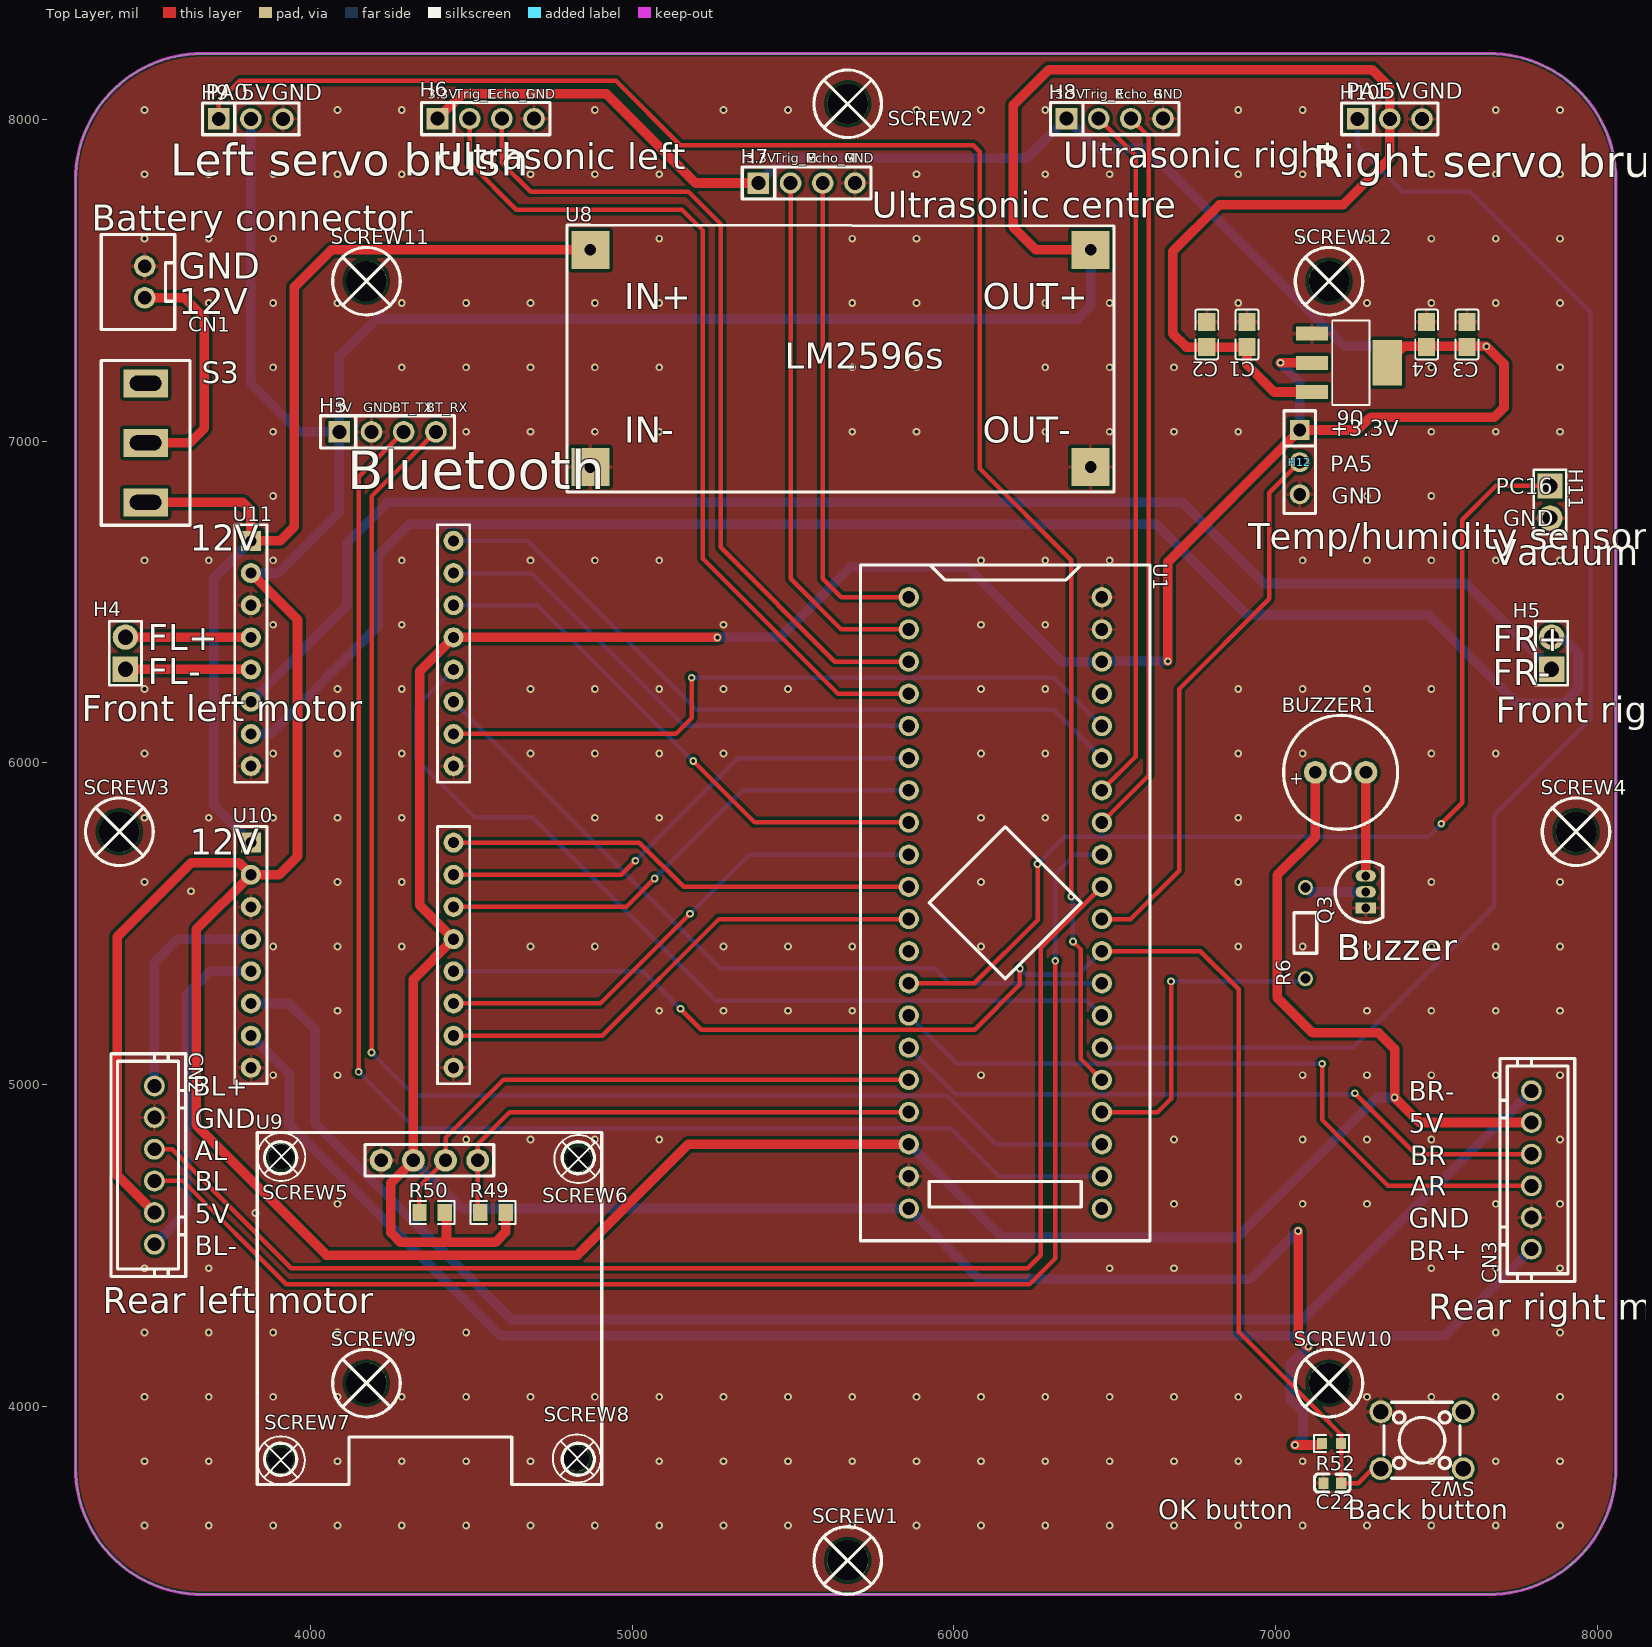
[diagram p0: Top Layer view]
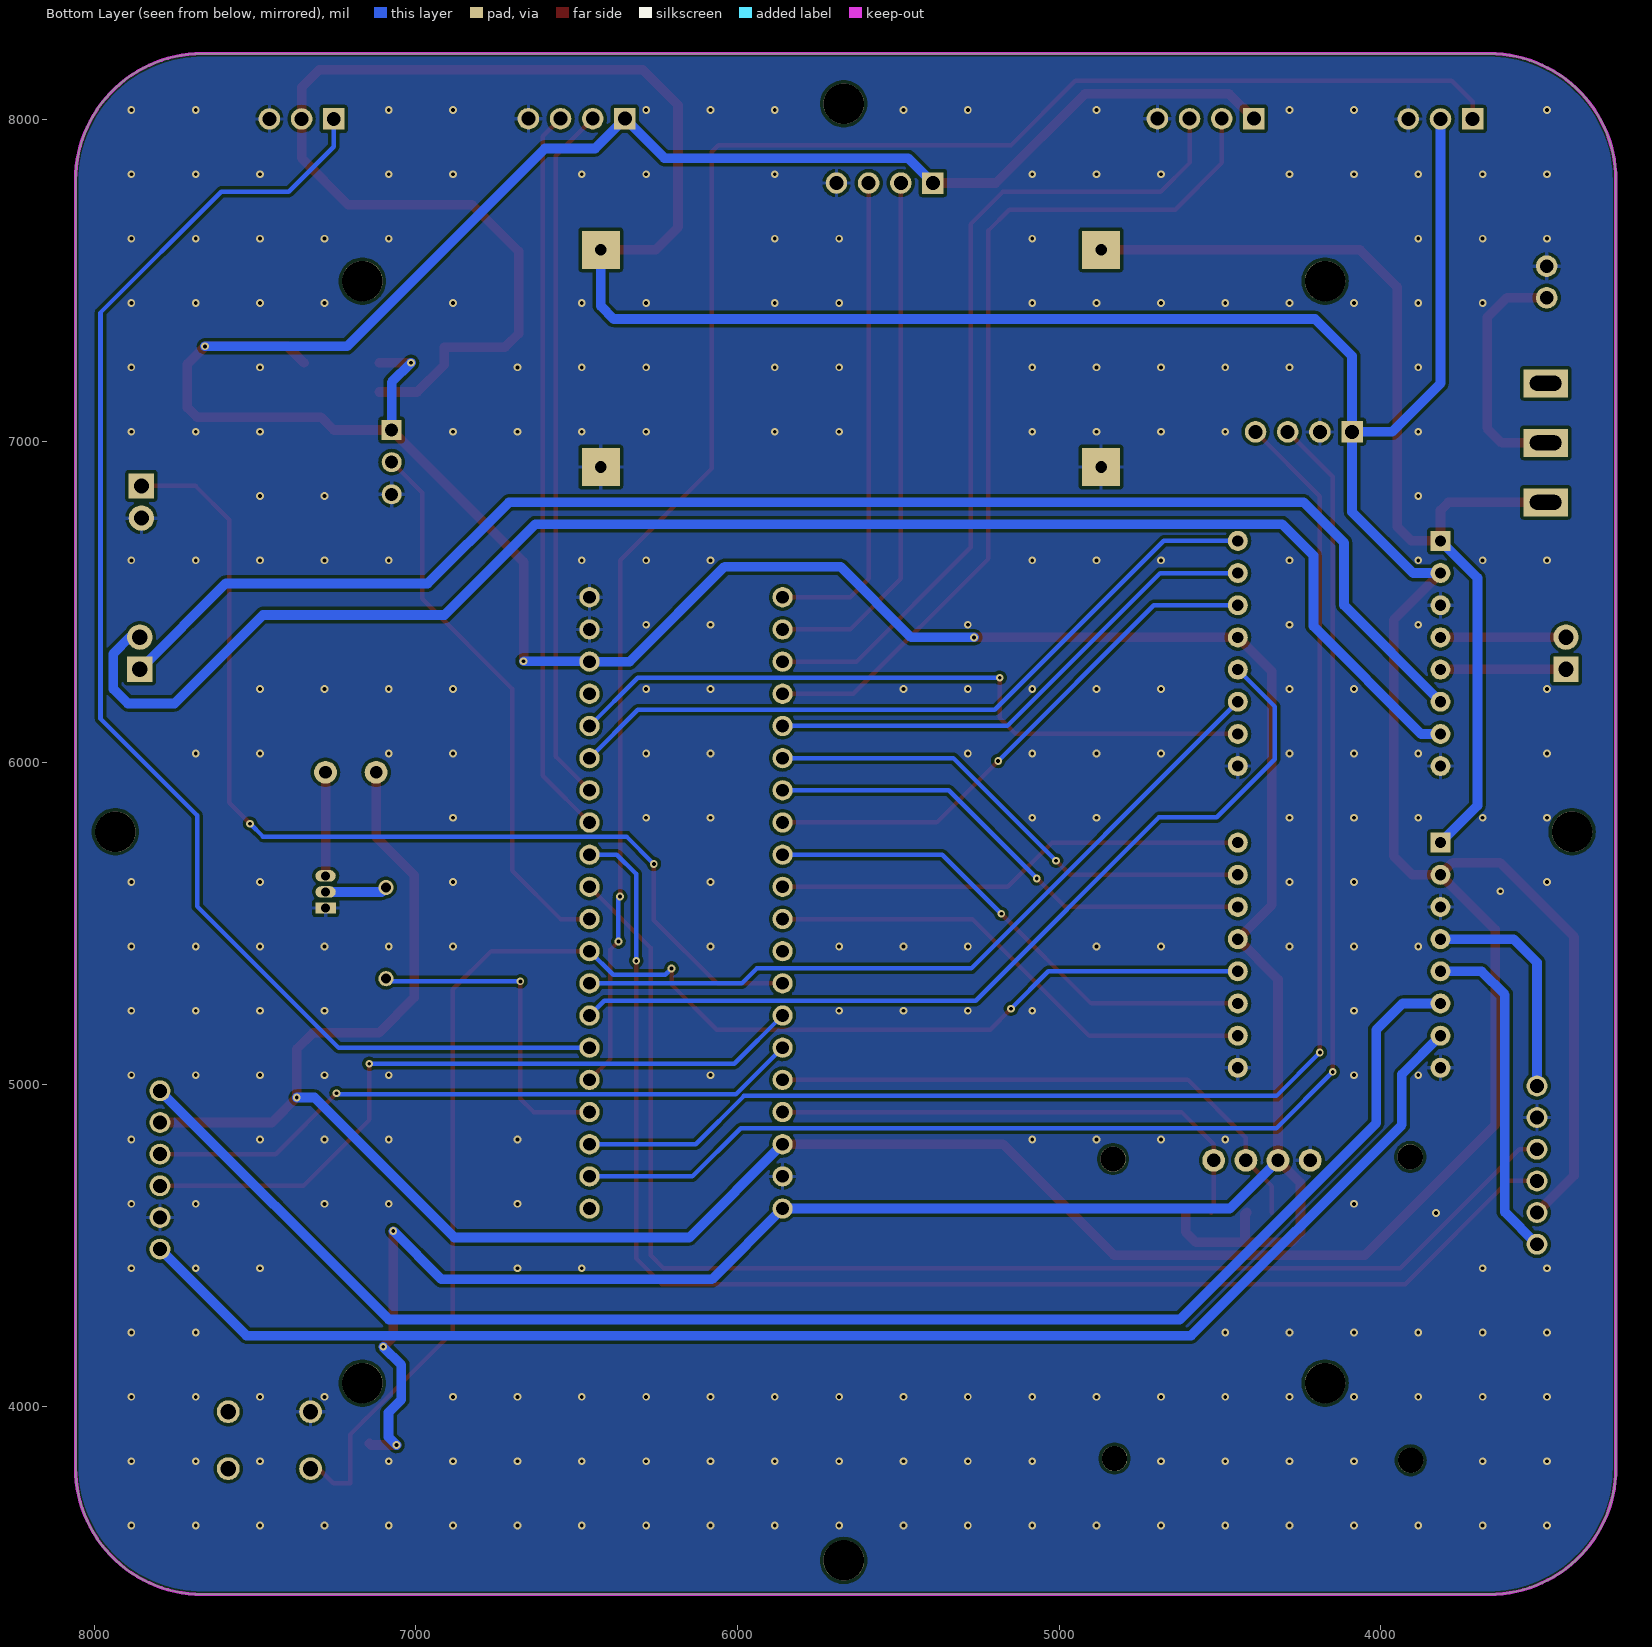
[diagram p1: Bottom Layer view, seen from below]
# Altium PCB MISC49897.pcbdoc
Units mil, origin at the board's own origin, x right, y up, seen from the top; angles counter-clockwise.
Board outline 4787.56 x 4789.41 mil, 2 copper layers (Top Layer, Bottom Layer), stack 62.206 mil thick; 44 components, 49 nets, 171 pads, 306 vias.

## Layer stack, top to bottom
Top Solder Mask Layer: solder mask 0.394, Dk 3.3
Top Layer: signal copper 1.379
Dielectric1: surface 59.449, FR4, Dk 4.5
Bottom Layer: signal copper 1.378
Bottom Solder Mask Layer: solder mask 0.394, Dk 3.3

## Board outline
3663.7,8205 ccw(c3663.7,7811.3) 3270,7811.3 3270,3809.29 ccw(c3663.7,3809.29) 3663.7,3415.59 7663.86,3415.59 ccw(c7663.86,3809.29) 8057.56,3809.29 8057.56,7811.3 ccw(c7663.86,7811.3) 7663.86,8205

## Design rules (kind name [scope] priority, off if disabled: settings)
BoardOutlineClearance copperThickness2oz_1 [All] p2 off: genericclearance=7.99 ignorepadtopadclearanceinfootprint=FALSE except(0: Arc-SplitContinuation Track-SplitContinuation SMDPad-SplitContinuation THPad-SplitContinuation Via-SplitContinuation Fill-SplitContinuation Region-SplitContinuation Poly-SplitContinuation Text-SplitContinuation Hole-SplitContinuation; 5.98: Arc-CutoutEdge Track-CutoutEdge SMDPad-CutoutEdge THPad-CutoutEdge Via-CutoutEdge Text-CutoutEdge; 6.9: Hole-OutlineEdge Hole-CutoutEdge; 10: Poly-OutlineEdge Poly-CutoutEdge; 11.81: Arc-OutlineEdge Track-OutlineEdge SMDPad-OutlineEdge THPad-OutlineEdge Via-OutlineEdge Fill-OutlineEdge Region-OutlineEdge Text-OutlineEdge Fill-CutoutEdge Region-CutoutEdge)
BoardOutlineClearance Plane_innerPlane_1 [All] p4 off: genericclearance=4.02 ignorepadtopadclearanceinfootprint=FALSE except(0: Arc-SplitContinuation Track-SplitContinuation SMDPad-SplitContinuation THPad-SplitContinuation Via-SplitContinuation Fill-SplitContinuation Region-SplitContinuation Poly-SplitContinuation Text-SplitContinuation Hole-SplitContinuation; 5.98: Arc-CutoutEdge Track-CutoutEdge SMDPad-CutoutEdge THPad-CutoutEdge Via-CutoutEdge Text-CutoutEdge; 6.9: Hole-OutlineEdge Hole-CutoutEdge; 10: Poly-OutlineEdge Poly-CutoutEdge; 11.81: Arc-OutlineEdge Track-OutlineEdge SMDPad-OutlineEdge THPad-OutlineEdge Via-OutlineEdge Fill-OutlineEdge Region-OutlineEdge Text-OutlineEdge Fill-CutoutEdge Region-CutoutEdge)
BoardOutlineClearance Copper_copperRegion_1 [All] p6 off: genericclearance=4.02 ignorepadtopadclearanceinfootprint=FALSE except(0: Arc-SplitContinuation Track-SplitContinuation SMDPad-SplitContinuation THPad-SplitContinuation Via-SplitContinuation Fill-SplitContinuation Region-SplitContinuation Poly-SplitContinuation Text-SplitContinuation Hole-SplitContinuation; 5.98: Arc-CutoutEdge Track-CutoutEdge SMDPad-CutoutEdge THPad-CutoutEdge Via-CutoutEdge Text-CutoutEdge; 6.9: Hole-OutlineEdge Hole-CutoutEdge; 10: Poly-OutlineEdge Poly-CutoutEdge; 11.81: Arc-OutlineEdge Track-OutlineEdge SMDPad-OutlineEdge THPad-OutlineEdge Via-OutlineEdge Fill-OutlineEdge Region-OutlineEdge Text-OutlineEdge Fill-CutoutEdge Region-CutoutEdge)
BoardOutlineClearance copperThickness1oz_1 [All] p8: genericclearance=4.02 ignorepadtopadclearanceinfootprint=FALSE except(0: Arc-SplitContinuation Track-SplitContinuation SMDPad-SplitContinuation THPad-SplitContinuation Via-SplitContinuation Fill-SplitContinuation Region-SplitContinuation Poly-SplitContinuation Text-SplitContinuation Hole-SplitContinuation; 5.98: Arc-CutoutEdge Track-CutoutEdge SMDPad-CutoutEdge THPad-CutoutEdge Via-CutoutEdge Text-CutoutEdge; 6.9: Hole-OutlineEdge Hole-CutoutEdge; 10: Poly-OutlineEdge Poly-CutoutEdge; 11.81: Arc-OutlineEdge Track-OutlineEdge SMDPad-OutlineEdge THPad-OutlineEdge Via-OutlineEdge Fill-OutlineEdge Region-OutlineEdge Text-OutlineEdge Fill-CutoutEdge Region-CutoutEdge)
Clearance copperThickness2oz [All] p1 off: gap=7.99 ignorepadtopadclearanceinfootprint=FALSE except(5.98: SMDPad-Track SMDPad-SMDPad THPad-Track SMDPad-THPad THPad-THPad Track-Via SMDPad-Via THPad-Via Via-Via Fill-SMDPad Region-SMDPad Fill-THPad Region-THPad Fill-Via Region-Via Fill-Fill Fill-Region Region-Region Arc-Track Arc-SMDPad Arc-THPad Arc-Via Fill-Arc Region-Arc Arc-Arc Text-Track SMDPad-Text Text-THPad Text-Via Fill-Text Region-Text Arc-Text Text-Text; 6.9: Hole-Track Hole-SMDPad Hole-THPad Hole-Via Fill-Hole Region-Hole Hole-Arc Hole-Text; 10: Poly-Track Poly-SMDPad Poly-THPad Poly-Via Poly-Fill Poly-Region Poly-Poly Poly-Arc Poly-Text Poly-Hole; 11.81: Fill-Track Region-Track)
Clearance Plane_innerPlane [All] p3 off: gap=4.02 ignorepadtopadclearanceinfootprint=FALSE except(5.98: SMDPad-Track SMDPad-SMDPad THPad-Track SMDPad-THPad THPad-THPad Track-Via SMDPad-Via THPad-Via Via-Via Fill-SMDPad Region-SMDPad Fill-THPad Region-THPad Fill-Via Region-Via Fill-Fill Fill-Region Region-Region Arc-Track Arc-SMDPad Arc-THPad Arc-Via Fill-Arc Region-Arc Arc-Arc Text-Track SMDPad-Text Text-THPad Text-Via Fill-Text Region-Text Arc-Text Text-Text; 6.9: Hole-Track Hole-SMDPad Hole-THPad Hole-Via Fill-Hole Region-Hole Hole-Arc Hole-Text; 10: Poly-Track Poly-SMDPad Poly-THPad Poly-Via Poly-Fill Poly-Region Poly-Poly Poly-Arc Poly-Text Poly-Hole; 11.81: Fill-Track Region-Track)
Clearance Copper_copperRegion [All] p5 off: gap=4.02 ignorepadtopadclearanceinfootprint=FALSE except(5.98: SMDPad-Track SMDPad-SMDPad THPad-Track SMDPad-THPad THPad-THPad Track-Via SMDPad-Via THPad-Via Via-Via Fill-SMDPad Region-SMDPad Fill-THPad Region-THPad Fill-Via Region-Via Fill-Fill Fill-Region Region-Region Arc-Track Arc-SMDPad Arc-THPad Arc-Via Fill-Arc Region-Arc Arc-Arc Text-Track SMDPad-Text Text-THPad Text-Via Fill-Text Region-Text Arc-Text Text-Text; 6.9: Hole-Track Hole-SMDPad Hole-THPad Hole-Via Fill-Hole Region-Hole Hole-Arc Hole-Text; 10: Poly-Track Poly-SMDPad Poly-THPad Poly-Via Poly-Fill Poly-Region Poly-Poly Poly-Arc Poly-Text Poly-Hole; 11.81: Fill-Track Region-Track)
Clearance copperThickness1oz [All] p7: gap=4.02 ignorepadtopadclearanceinfootprint=FALSE except(5.98: SMDPad-Track SMDPad-SMDPad THPad-Track SMDPad-THPad THPad-THPad Track-Via SMDPad-Via THPad-Via Via-Via Fill-SMDPad Region-SMDPad Fill-THPad Region-THPad Fill-Via Region-Via Fill-Fill Fill-Region Region-Region Arc-Track Arc-SMDPad Arc-THPad Arc-Via Fill-Arc Region-Arc Arc-Arc Text-Track SMDPad-Text Text-THPad Text-Via Fill-Text Region-Text Arc-Text Text-Text; 6.9: Hole-Track Hole-SMDPad Hole-THPad Hole-Via Fill-Hole Region-Hole Hole-Arc Hole-Text; 10: Poly-Track Poly-SMDPad Poly-THPad Poly-Via Poly-Fill Poly-Region Poly-Poly Poly-Arc Poly-Text Poly-Hole; 11.81: Fill-Track Region-Track)
DiffPairsRouting differentialPair [All] p1: maxlimit=6 minlimit=6 mostfreqgap=6 toplayer_minwidth=5 toplayer_prefwidth=10 toplayer_maxwidth=100 toplayer_mingap=6 toplayer_prefgap=6 toplayer_maxgap=6 bottomlayer_minwidth=5 bottomlayer_prefwidth=10 bottomlayer_maxwidth=100 bottomlayer_mingap=6 bottomlayer_prefgap=6 bottomlayer_maxgap=6 maxuncoupledlength=10
HoleToHoleClearance otherClearance [All] p1: gap=11.81 allowstackedmicrovias=TRUE
Length netLength [All] p1: minlimit=0 maxlimit=0
PasteMaskExpansion pasteMaskExpansion [All] p1: expansion=0
PlaneConnect innerPlane [All] p1: planeconnectstyle=Relief reliefexpansion=20 reliefentries=4 reliefconductorwidth=10 reliefairgap=10
PolygonConnect copperRegion [All] p1: connectstyle=Relief reliefconductorwidth=10 reliefentries=4 polygonreliefangle="90 Angle" airgapwidth=10 via.connectstyle=Relief via.reliefconductorwidth=10 via.reliefentries=4 via.polygonreliefangle="90 Angle" via.airgapwidth=10
RoutingVias viaSize [All] p1: holewidth=12.01 width=24.02 viastyle="Through Hole" minholewidth=11.81 minwidth=19.68 maxholewidth=248.03 maxwidth=393.7
SolderMaskExpansion solderMaskExpansion [IsVia] p1: expansion=-1000 istentingtop=TRUE
SolderMaskExpansion solderMaskExpansion [All] p2: expansion=2 istentingtop=FALSE
Width copperThickness2oz_2 [All] p1 off: maxlimit=100 minlimit=8 preferedwidth=10
Width copperThickness1oz_2 [All] p2: maxlimit=100 minlimit=5 preferedwidth=10

## Components (designator, comment, footprint, x,y, rotation, side; value= is the part's Value field where it differs from the comment)
BUZZER1 "2.7kHz" BUZ-TH_BD9.0-P4.00-D0.6-FD 7202.04,5970.88 r0 top
C1 "10uF" C0805 6911.05,7331.73 r270 top
C2 "100nF" C0805 6786.05,7331.73 r270 top
C3 "10uF" C0805 7595,7331.73 r270 top
C4 "100nF" C0805 7469.55,7331.73 r270 top
C22 "1uF" C0603 7176.51,3761.54 r0 top
CN1 "XH2.54*2P_THT" CONN-TH_2P-P2.50-XH2.54-2P 3485,7495 r270 top
CN2 "Rear left motor" CONN-TH_XH2.54-6P 3515,4750.06 r270 top
CN3 "Rear right motor" CONN-TH_XH2.54-6P 7795,4735 r90 top
H3 "2.54-1*4P female" HDR-TH_4P-P2.54-V-F 4240,7029.1 r0 top
H4 "Front left motor" HDR-TH_2P-P2.54-V-M 3425,6340.99 r90 top
H5 "Front right motor" HDR-TH_2P-P2.54-V-M 7857.83,6340.99 r90 top
H6 "Ultrasonic left" HDR-TH_4P-P2.54-V-M 4544.98,8002.56 r0 top
H7 "Ultrasonic centre" HDR-TH_4P-P2.54-V-M 5542.5,7802.56 r0 top
H8 "Ultrasonic right" HDR-TH_4P-P2.54-V-M 6500.02,8002.56 r0 top
H9 "PZ254V-11-03P" HDR-TH_3P-P2.54-V-M 3815,8001.77 r0 top
H10 "PZ254V-11-03P" HDR-TH_3P-P2.54-V-M 7355,8001.77 r0 top
H11 "PZ254V-11-02P" HDR-TH_2P-P2.54-V-M 7852.83,6810.94 r270 top
H12 "PM254V-11-03-H85" HDR-TH_3P-P2.54-V-F 7075,6935 r270 top
Q3 "" S8050_TO_92 7280.18,5599.13 r90 top
R6 "1K" Res_1/8W 7095,5471.23 r90 top
R49 "4.7kΩ" R0805 4567.58,4602.68 r180 top
R50 "4.7kΩ" R0805 4378.22,4602.68 r180 top
R52 "10kΩ" R0603 7173.71,3885 r180 top
S3 "SS12D10 switch" SS12D10 3487.96,6810 r90 top
SCREW1 "" M3螺丝 5670,3521.23 r0 top
SCREW2 "" M3螺丝 5670,8048.77 r0 top
SCREW3 "" M3螺丝 3406.22,5786.33 r0 top
SCREW4 "" M3螺丝 7933.78,5786.33 r0 top
SCREW5 "" M2螺丝 3909.2,4775.46 r0 top
SCREW6 "" M2螺丝 4832.85,4768.94 r0 top
SCREW7 "" M2螺丝 3907.97,3832.39 r0 top
SCREW8 "" M2螺丝 4828.16,3838.02 r0 top
SCREW9 "" M3螺丝 4173.96,4072.42 r0 top
SCREW10 "" M3螺丝 7166.08,4072.42 r0 top
SCREW11 "" M3螺丝 4173.96,7497.58 r0 top
SCREW12 "" M3螺丝 7166.08,7497.58 r0 top
SW2 "" SW-TH_4P-L6.0-W6.0-P4.50-LS6.5 7455,3895 r180 top
U1 "STM32F103C8T6-Card" CONN-TH_L53.3-W22.9_STM32F103C8T6-CARD 6160,5565 r270 top
U6 "AMS1117-3.3" SOT-223-3_L6.5-W3.4-P2.30-LS7.0-BR 7230,7243.77 r180 top
U8 "LM2596S buck module" LM2596S 4870,7595 r0 top
U9 "HS96L03W2C03" OLED-TH_L27.8-W27.2-P2.54_C9900033791 4370,4765 r0 top
U10 "TB6612 module" TB6612-2X8 3815,5752.44 r0 top
U11 "TB6612 module" TB6612-2X8 3815,6690.26 r0 top

## Footprints (in the part's own frame and the unit in brackets; to place one, negate y for a bottom-side part, rotate by r counter-clockwise, add the part's x,y. Pads: shape width x height; smd on the part's side, far side on the other; paste and mask are expansions set on the pad)
BUZ-TH_BD9.0-P4.00-D0.6-FD [mm]
  round 1.8 hole 1: 1(-2,0) 2(2,0)
  silkscreen extent -4.5,-4.5 4.5,4.5
C0603 [mm]
  rect 0.8x0.9 smd paste+0 mask+0.051: 1(-0.7,0) 2(0.7,0)
  silkscreen extent -1.41,-0.71 1.39,0.72
C0805 [mm]
  rect 1.41x1.35 smd paste-100 mask+0.051: 1(-1,0) 2(1,0)
  silkscreen extent -1.96,-0.9 1.96,0.9
CONN-TH_2P-P2.50-XH2.54-2P [mm]
  round 1.7 hole 1.05 paste+0 mask+0.05: 1(1.25,0) 2(-1.25,0)
  silkscreen extent -3.75,-3.42 3.75,2.37
CONN-TH_L53.3-W22.9_STM32F103C8T6-CARD [mm]
  round 1.6 hole 1: 1(-24.13,-7.62) 2(-21.59,-7.62) 3(-19.05,-7.62) 4(-16.51,-7.62) 5(-13.97,-7.62) 6(-11.43,-7.62) 7(-8.89,-7.62) 8(-6.35,-7.62) 9(-3.81,-7.62) 10(-1.27,-7.62) 11(1.27,-7.62) 12(3.81,-7.62) 13(6.35,-7.62) 14(8.89,-7.62) 15(11.43,-7.62) 16(13.97,-7.62) 17(16.51,-7.62) 18(19.05,-7.62) 19(21.59,-7.62) 20(24.13,-7.62) 21(24.13,7.62) 22(21.59,7.62) 23(19.05,7.62) 24(16.51,7.62) 25(13.97,7.62) 26(11.43,7.62) 27(8.89,7.62) 28(6.35,7.62) 29(3.81,7.62) 30(1.27,7.62) 31(-1.27,7.62) 32(-3.81,7.62) 33(-6.35,7.62) 34(-8.89,7.62) 35(-11.43,7.62) 36(-13.97,7.62) 37(-16.51,7.62) 38(-19.05,7.62) 39(-21.59,7.62) 40(-24.13,7.62)
  silkscreen extent -26.67,-11.43 26.67,11.43
CONN-TH_XH2.54-6P [mm]
  round 1.65 hole 1.1 paste+0 mask+0.05: 1(-6.25,0) 2(-3.75,0) 3(-1.25,0) 4(1.25,0) 5(3.75,0) 6(6.25,0)
  silkscreen extent -8.8,-3.43 8.8,2.47
HDR-TH_2P-P2.54-V-M [mm]
  rect 2x2 hole 1.2: 1(-1.27,0)
  round 2 hole 1.2: 2(1.27,0)
  silkscreen extent -2.54,-1.27 2.54,1.27
HDR-TH_3P-P2.54-V-F [mil]
  rect 62x62 hole 40.16: 1(-100,0)
  round 62 hole 40.16: 2(0,0) 3(100,0)
  silkscreen extent -160,-49 160,49
HDR-TH_3P-P2.54-V-M [mm]
  rect 1.7x1.7 hole 1.1: 1(-2.54,0)
  round 1.7 hole 1.1: 2(0,0) 3(2.54,0)
  silkscreen extent -3.81,-1.25 3.81,1.25
HDR-TH_4P-P2.54-V-F [mm]
  rect 1.7x1.7 hole 1.1: 1(-3.81,0)
  round 1.7 hole 1.1: 2(-1.27,0) 3(1.27,0) 4(3.81,0)
  silkscreen extent -5.29,-1.27 5.29,1.27
HDR-TH_4P-P2.54-V-M [mm]
  rect 1.7x1.7 hole 1.1: 1(-3.81,0)
  round 1.7 hole 1.1: 2(-1.27,0) 3(1.27,0) 4(3.81,0)
  silkscreen extent -5.08,-1.27 5.08,1.27
LM2596S [mm]
  rect 3x3 hole 0.914 paste+0 mask+0.102: 1(0,0) 2(0,-17.145) 3(39.497,-17.145) 4(39.497,0)
  silkscreen extent -1.84,-19.11 41.34,1.97
M2螺丝 [mm]
  round 2 hole 2: 1(0,0)
  silkscreen extent -1.9,-1.9 1.9,1.9
M3螺丝 [mil]
  round 126 hole 126 paste+0 mask+4: 1(0,0)
  silkscreen extent -105,-105 105,105
OLED-TH_L27.8-W27.2-P2.54_C9900033791 [mm]
  round 1.8 hole 1.05 paste+0 mask+0.05: 1(-3.81,0) 2(-1.27,0) 3(1.27,0) 4(3.81,0)
  silkscreen extent -13.6,-25.6 13.6,2.2
R0603 [mil]
  rect 31.75x34.02 smd paste-3937.01 mask+2: 1(-29.66,0) 2(29.66,0)
  silkscreen extent -55,-26 55,26
R0805 [mm]
  rect 1.133x1.377 smd paste-100 mask+0.051: 1(-1,0) 2(1,0)
  silkscreen extent -1.76,-0.92 1.76,0.92
Res_1/8W [mil]
  round 47.2 hole 31.5 paste+0 mask+2: 1(-141.7,2.48) 2(141.7,2.48)
  silkscreen extent -63,-33 63,38
S8050_TO_92 [mil]
  rect 35.4x63 hole 27.6 paste+0 mask+2: 1(-50,0)
  oval 35.4x63 hole 27.6 paste+0 mask+2: 2(0,0) 3(50,0)
  silkscreen extent -95,-53 95,95
SOT-223-3_L6.5-W3.4-P2.30-LS7.0-BR [mm]
  rect 2.5x1.1 smd: 1(2.97,-2.3) 2(2.97,0) 3(2.97,2.3)
  rect 2.34x3.6 smd: 4(-2.97,0)
  silkscreen extent -1.57,-3.33 1.37,3.33
SS12D10 [mil]
  rect 86.6x137.8 hole 47.2 slot 98.4 at 90 deg paste+0 mask+4: 1(0,0) 2(185,0) 3(370,0)
  silkscreen extent -71,-138 441,138
SW-TH_4P-L6.0-W6.0-P4.50-LS6.5 [mm]
  round 1.8 hole 1.2: 1(-3.25,2.25) 2(3.25,2.25) 3(-3.25,-2.25) 4(3.25,-2.25)
  silkscreen extent -3,-3 3,3
TB6612-2X8 [mil]
  rect 62x62 hole 35: 1(0,0)
  round 62 hole 35: 2(0,-100) 3(0,-200) 4(0,-300) 5(0,-400) 6(0,-500) 7(0,-600) 8(0,-700) 9(629.92,-700) 10(629.92,-600) 11(629.92,-500) 12(629.92,-400) 13(629.92,-300) 14(629.92,-200) 15(629.92,-100) 16(629.92,0)
  silkscreen extent -50,-750 680,50

## Via types
v1: diameter 24.02, hole 12, Top Layer to Bottom Layer, 306 vias

## Nets (pads, with @x,y where several pads share a name; then routed paths per layer and width w, separated by ;. In a path a pad name is that pad's centre, name@x,y a point inside that pad or via, vN(x,y) a via of type N, cw(c..) or ccw(c..) an arc to the next point about the centre after c; other vN are vias at no path point)
$1N3770: CN1.1 S3.2 | length 755.9
  Top Layer w30: CN1.1 3609.21,7445.79 3670,7385 3670,7040 3625,6995 S3.2
$1N10272: Q3.2 R6.2 | length 193.4
  Bottom Layer w30: R6.2 7106.33,5599.13 Q3.2
$1N10274: BUZZER1.2 Q3.3 | length 322
  Top Layer w30: Q3.3 7280.18,5970.28 BUZZER1.2
+3.3V: C3.2 C4.2 H6.1 H7.1 H8.1 H12.1 R49.1 R50.1 R52.2 U1.20 U1.38 U6.2 U6.4 U9.2 U10.13 U11.13 | length 14979.3
  Top Layer w30: H6.1 4472.42,8080 4920,8080 5197.44,7802.56 H7.1 ; R50.1 4422.79,4597.48 4422.79,4510 ; R49.1 4606.95,4541.95 4575,4510 4422.79,4510 ; v1(5264.74,6390.26) U11.13 4340,6285.34 4340,5557.36 U10.13 4320,5327.52 U9.2 4250,4695 4250,4540 4280,4510 4422.79,4510 ; v1(6665,6316.23) 6665,6625 H12.1 7075,7034.77 7255,7034.77 7295.23,7075 7680,7075 7710,7105 7710,7240 v1(7655,7295) 7398.16,7295 U6.4 ; v1(7015,7243.77) U6.2 ; v1(7060,3880) 7139.05,3880 R52.2 ; v1(7070,4545) 7070,4216.79 v1(7101.38,4185.41)
  Bottom Layer w30: U9.2 4470,4615 U1.20 6080,4395 6920,4395 v1(7070,4545) ; v1(5264.74,6390.26) 5460.26,6390.26 5680,6610 6040,6610 6335,6315 U1.38 6461.23,6316.23 v1(6665,6316.23) ; H7.1 5469.94,7880 6227.46,7880 H8.1 6442.58,7910 6598.77,7910 7213.77,7295 v1(7655,7295) ; v1(7015,7243.77) 7075,7183.77 H12.1 ; v1(7060,3880) 7085,3905 7085,3981.23 7045,4021.23 7045,4129.03 v1(7101.38,4185.41)
+5V: BUZZER1.1 C1.2 C2.2 CN2.5 CN3.5 H3.1 H9.2 H10.2 U1.18 U6.3 U8.4 U10.2 U11.2 | length 17782.1
  Top Layer w30: CN2.5 3400,4717.42 3400,5460 3630,5690 3777.44,5690 U10.2 ; U11.2 3960,6445.26 3960,5710 3902.44,5652.44 U10.2 ; U1.18 5175,4815 4830,4470 4050,4470 3645,4875 3645,5482.44 U10.2 ; U8.4 6255,7595 6185,7665 6185,8045 6295,8155 7300,8155 7355,8100 H10.2 7355,7880 7210,7735 6825,7735 6680,7590 6680,7335 6722.64,7292.36 C2.2 C1.2 6911.05,7237.72 6995.55,7153.22 U6.3 ; BUZZER1.1 7123.3,5769.53 7005,5651.23 7005,5271.23 7115,5161.23 7320,5161.23 7370,5111.23 v1(7370,4960) 7447.36,4882.64 CN3.5
  Bottom Layer w30: U11.2 3900.26,6590.26 4090,6780 H3.1 ; H9.2 3815,7180 3965.9,7029.1 H3.1 ; U1.18 6150,4525 6880,4525 7315,4960 v1(7370,4960) ; U8.4 6425,7420 6385,7380 4205,7380 4090,7265 H3.1
AL: CN2.3 U1.31 | length 4148.2
  Top Layer w14: CN2.3 3570.73,4799.27 3940,4430 6230,4430 6270,4470 6270,5425 U1.31
AR: CN3.3 U1.14 | length 2256.5
  Top Layer w14: v1(7144.69,5065) 7144.69,4890.31 7349.21,4685.79 CN3.3
  Bottom Layer w14: U1.14 6010,5065 v1(7144.69,5065)
BL: CN2.4 U1.32 | length 4330.9
  Top Layer w14: CN2.4 3604.15,4700.85 3925,4380 6235,4380 6315,4460 v1(6315,5385)
  Bottom Layer w14: v1(6315,5385) 6315,5655 6375,5715 U1.32
BR: CN3.4 U1.15 | length 2075
  Top Layer w14: v1(7246.38,4973.62) 7435.79,4784.21 CN3.4
  Bottom Layer w14: U1.15 6005,4970 7242.77,4970 v1(7246.38,4973.62)
BT_RX: H3.4 U1.23 | length 4400
  Top Layer w14: v1(4190,5100) 4190,6829.1 H3.4
  Bottom Layer w14: v1(4190,5100) 4325,4965 5980,4965 6130,4815 U1.23
BT_TX: H3.3 U1.22 | length 4491.7
  Top Layer w14: v1(4150,5040) 4150,6889.1 H3.3
  Bottom Layer w14: v1(4150,5040) 4325,4865 5990,4865 6140,4715 U1.22
ECHO_L: H6.3 U1.3 | length 2633.3
  Top Layer w14: H6.3 4594.98,7865.02 4685,7775 5175,7775 5275,7675 5275,6670 5630,6315 U1.3
ECHO_M: H7.3 U1.1 | length 1521.4
  Top Layer w14: H7.3 5592.5,6572.5 5650,6515 U1.1
ECHO_R: H8.3 U1.33 | length 2270.4
  Top Layer w14: U1.33 6605,5960 6605,7947.58 H8.3
GND: C1.1 C2.1 C3.1 C4.1 C22.1 CN1.2 CN2.2 CN3.2 H3.2 H6.4 H7.4 H8.4 H9.3 H10.3 H11.2 H12.3 Q3.1 SW2.4 U1.19 U1.39 U1.40 U6.1 U8.2 U8.3 U9.1 U10.3 U10.8 U10.9 U11.3 U11.8 U11.9
  other v1: 3484.1,3629.69 3684.1,3629.69 3884.1,3629.69 4084.1,3629.69 4284.1,3629.69 4484.1,3629.69 4684.1,3629.69 4884.1,3629.69 5084.1,3629.69 5284.1,3629.69 5484.1,3629.69 5684.1,3629.69 5884.1,3629.69 6084.1,3629.69 6284.1,3629.69 6484.1,3629.69 6684.1,3629.69 6884.1,3629.69 7084.1,3629.69 7284.1,3629.69 7484.1,3629.69 7684.1,3629.69 7884.1,3629.69 3484.1,3829.69 3684.1,3829.69 4084.1,3829.69 4284.1,3829.69 4484.1,3829.69 4684.1,3829.69 5084.1,3829.69 5284.1,3829.69 5484.1,3829.69 5684.1,3829.69 5884.1,3829.69 6084.1,3829.69 6284.1,3829.69 6484.1,3829.69 6684.1,3829.69 6884.1,3829.69 7084.1,3829.69 7484.1,3829.69 7684.1,3829.69 7884.1,3829.69 3484.1,4029.69 3684.1,4029.69 3884.1,4029.69 4084.1,4029.69 4284.1,4029.69 4484.1,4029.69 4684.1,4029.69 4884.1,4029.69 5084.1,4029.69 5284.1,4029.69 5484.1,4029.69 5684.1,4029.69 5884.1,4029.69 6084.1,4029.69 6284.1,4029.69 6484.1,4029.69 6684.1,4029.69 6884.1,4029.69 7284.1,4029.69 7484.1,4029.69 7684.1,4029.69 7884.1,4029.69 3484.1,4229.69 3684.1,4229.69 3884.1,4229.69 4084.1,4229.69 4284.1,4229.69 4484.1,4229.69 7684.1,4229.69 7884.1,4229.69 3484.1,4429.69 3684.1,4429.69 6484.1,4429.69 6684.1,4429.69 7484.1,4429.69 7684.1,4429.69 7884.1,4429.69 3829.1,4601.1 4084.1,4629.69 6684.1,4629.69 7084.1,4629.69 7284.1,4629.69 7684.1,4629.69 7884.1,4629.69 4484.1,4829.69 4684.1,4829.69 4884.1,4829.69 5084.1,4829.69 6684.1,4829.69 7084.1,4829.69 7284.1,4829.69 7484.1,4829.69 7884.1,4829.69 3884.1,5029.69 4084.1,5029.69 6084.1,5029.69 7084.1,5029.69 7284.1,5029.69 7484.1,5029.69 7684.1,5029.69 7884.1,5029.69 4084.1,5229.69 5084.1,5229.69 5284.1,5229.69 5484.1,5229.69 5684.1,5229.69 7284.1,5229.69 7484.1,5229.69 7684.1,5229.69 7884.1,5229.69 3884.1,5429.69 4084.1,5429.69 4284.1,5429.69 4684.1,5429.69 4884.1,5429.69 5284.1,5429.69 5484.1,5429.69 5684.1,5429.69 6084.1,5429.69 6884.1,5429.69 7084.1,5429.69 7284.1,5429.69 7484.1,5429.69 7684.1,5429.69 7884.1,5429.69 3629.1,5601.1 3484.1,5629.69 4084.1,5629.69 4284.1,5629.69 6084.1,5629.69 6884.1,5629.69 7484.1,5629.69 7884.1,5629.69 3484.1,5829.69 3684.1,5829.69 3884.1,5829.69 4084.1,5829.69 4284.1,5829.69 4884.1,5829.69 5084.1,5829.69 6084.1,5829.69 6284.1,5829.69 6884.1,5829.69 3484.1,6029.69 3884.1,6029.69 4084.1,6029.69 4284.1,6029.69 4684.1,6029.69 4884.1,6029.69 5084.1,6029.69 5284.1,6029.69 6084.1,6029.69 6284.1,6029.69 6884.1,6029.69 7084.1,6029.69 7484.1,6029.69 7684.1,6029.69 3484.1,6229.69 4084.1,6229.69 4284.1,6229.69 4684.1,6229.69 4884.1,6229.69 5084.1,6229.69 5284.1,6229.69 5484.1,6229.69 6084.1,6229.69 6284.1,6229.69 6884.1,6229.69 7084.1,6229.69 7284.1,6229.69 7484.1,6229.69 3884.1,6429.69 4284.1,6429.69 5284.1,6429.69 6084.1,6429.69 6284.1,6429.69 3484.1,6629.69 3684.1,6629.69 3884.1,6629.69 4284.1,6629.69 4684.1,6629.69 4884.1,6629.69 5084.1,6629.69 6084.1,6629.69 6284.1,6629.69 6484.1,6629.69 7084.1,6629.69 7284.1,6629.69 7484.1,6629.69 7684.1,6629.69 7884.1,6629.69 3884.1,6829.69 7284.1,6829.69 7484.1,6829.69 3884.1,7029.69 4484.1,7029.69 4684.1,7029.69 4884.1,7029.69 5084.1,7029.69 5684.1,7029.69 5884.1,7029.69 6284.1,7029.69 6484.1,7029.69 6684.1,7029.69 6884.1,7029.69 7484.1,7029.69 7684.1,7029.69 7884.1,7029.69 3884.1,7229.69 4284.1,7229.69 4484.1,7229.69 4684.1,7229.69 4884.1,7229.69 5084.1,7229.69 5684.1,7229.69 5884.1,7229.69 6284.1,7229.69 6484.1,7229.69 6684.1,7229.69 7484.1,7229.69 7884.1,7229.69 3684.1,7429.69 3884.1,7429.69 4084.1,7429.69 4284.1,7429.69 4484.1,7429.69 4684.1,7429.69 4884.1,7429.69 5084.1,7429.69 5684.1,7429.69 5884.1,7429.69 6284.1,7429.69 6484.1,7429.69 6884.1,7429.69 7284.1,7429.69 7484.1,7429.69 7684.1,7429.69 7884.1,7429.69 3484.1,7629.69 3684.1,7629.69 3884.1,7629.69 5084.1,7629.69 5684.1,7629.69 5884.1,7629.69 7084.1,7629.69 7284.1,7629.69 7484.1,7629.69 7684.1,7629.69 7884.1,7629.69 3484.1,7829.69 3684.1,7829.69 3884.1,7829.69 4084.1,7829.69 4284.1,7829.69 4684.1,7829.69 4884.1,7829.69 5084.1,7829.69 5884.1,7829.69 6284.1,7829.69 6484.1,7829.69 6884.1,7829.69 7084.1,7829.69 7484.1,7829.69 7684.1,7829.69 7884.1,7829.69 3484.1,8029.69 4084.1,8029.69 4284.1,8029.69 4884.1,8029.69 5284.1,8029.69 5484.1,8029.69 5884.1,8029.69 6084.1,8029.69 6284.1,8029.69 6884.1,8029.69 7084.1,8029.69 7684.1,8029.69 7884.1,8029.69
L+: H4.2 U11.4 | length 390.3
  Top Layer w30: H4.2 3814.27,6390.99 U11.4
L-: H4.1 U11.5 | length 390.3
  Top Layer w30: H4.1 3814.27,6290.99 U11.5
ML+: CN2.1 U10.4 | length 713.9
  Bottom Layer w30: CN2.1 3515,5380 3587.44,5452.44 U10.4
ML-: CN2.6 U10.5 | length 1047.4
  Bottom Layer w30: CN2.6 3615,4604 3615,5280 3687.44,5352.44 U10.5
MR+: CN3.1 U10.7 | length 4569.9
  Bottom Layer w30: U10.7 3935,5032.44 3935,4875 4590,4220 7526.06,4220 CN3.1
MR-: CN3.6 U10.6 | length 4851.3
  Bottom Layer w30: U10.6 3932.56,5252.44 4015,5170 4015,4880 4625,4270 7083.94,4270 CN3.6
NRST: U1.37
OLED_SCL: R50.2 U1.16 U9.3 | length 1780.5
  Top Layer w14: R50.2 4338.85,4683.85 U9.3 4420,4835 4600,5015 U1.16
OLED_SDA: R49.2 U1.17 U9.4 | length 1597.1
  Top Layer w14: R49.2 4520,4610.89 U9.4 4520,4815 4620,4915 U1.17
PA0: H9.1 U1.25 | length 5578.7
  Top Layer w14: H9.1 3715,8055 3780,8120 4950,8120 5150,7920 6060,7920 6080,7900 6080,6915 6365,6630 v1(6365,5585) ; v1(6370,5445) 6395,5420 6395,5080 U1.25
  Bottom Layer w14: v1(6365,5585) 6370,5580 v1(6370,5445)
PA1: H10.1 U1.26 | length 4396.6
  Bottom Layer w14: U1.26 7240,5115 7680,5555 7680,5837.25 7980,6137.25 7980,7400 7605,7775 7395,7775 7255,7915 H10.1
PA2: U1.27 U11.12 | length 2786.4
  Bottom Layer w14: U11.12 4330,6175.34 4330,6011.23 4510,5831.23 4690,5831.23 5260,5261.23 6413.77,5261.23 U1.27
PA3: U1.28 U11.11 | length 2377.6
  Bottom Layer w14: U11.11 5273.95,5361.23 5940,5361.23 5986.23,5315 U1.28
PA4: C22.2 R52.1 SW2.2 U1.29 U10.12 | length 4520.5
  Top Layer w14: v1(5150,5236.23) 5215,5171.23 5840.87,5171.23 5841.58,5170.52 5878.43,5170.52 5879.14,5171.23 6065,5171.23 6205,5311.23 v1(6205,5361.23) ; U1.29 6766.23,5415 6885,5296.23 6885,4231.23 7150.21,3966.02 7150.78,3966.02 7166.02,3950.78 7166.02,3950.21 7203.37,3912.86 R52.1 7204.07,3884.3 C22.2 7256.54,3761.54 7301.42,3806.42 SW2.2
  Bottom Layer w14: U10.12 5033.79,5352.44 v1(5150,5236.23) ; v1(6205,5361.23) 6225,5341.23 6386.23,5341.23 U1.29
PA5: H12.2 U1.30 | length 1701.4
  Top Layer w14: U1.30 6550,5515 6700,5665 6700,6230 6980,6510 6980,6840 H12.2@7056.6,6916.6
PA8: U1.5 U11.15 | length 1611.9
  Bottom Layer w14: U11.15 4685.97,6590.26 5161.23,6115 U1.5
PA9: U1.6 U10.15 | length 1565.3
  Top Layer w14: U10.15 4966.21,5652.44 v1(5010,5696.23)
  Bottom Layer w14: v1(5010,5696.23) 5328.77,6015 U1.6
PA10: U1.7 U10.14 | length 1565.3
  Top Layer w14: U10.14 4981.21,5552.44 v1(5070,5641.23)
  Bottom Layer w14: v1(5070,5641.23) 5343.77,5915 U1.7
PA11: U1.8 U11.14 | length 1694.8
  Top Layer w14: v1(5190,6006.23) 5381.23,5815 U1.8
  Bottom Layer w14: U11.14 4705.97,6490.26 v1(5190,6006.23)
PA12: U1.9 U10.11 | length 1606.7
  Top Layer w14: U10.11 4901.21,5252.44 v1(5180,5531.23)
  Bottom Layer w14: v1(5180,5531.23) 5363.77,5715 U1.9
PA15: U1.10 U10.16 | length 1472
  Top Layer w14: U10.16 5022.56,5752.44 5160,5615 U1.10
PB1: H8.2 U1.34 | length 2178.7
  Top Layer w14: H8.2 6565,7887.58 6565,6020 U1.34
PB3: U1.11 U10.10 | length 1565.3
  Top Layer w14: U10.10 4907.44,5152.44 5270,5515 U1.11
PB4: U1.12
PB5: H11.1 U1.13 | length 3251.8
  Top Layer w14: U1.13 6063.77,5315 6260,5511.23 v1(6260,5686.23) ; v1(7515,5811.23) 7580,5876.23 7580,6756.23 7684.72,6860.94 H11.1
  Bottom Layer w14: v1(6260,5686.23) 6345,5771.23 6440.87,5771.23 6441.58,5770.52 6478.43,5770.52 6479.14,5771.23 7475,5771.23 v1(7515,5811.23)
PB10: U1.35 U11.16 | length 2294.8
  Bottom Layer w14: U11.16 4674.74,6690.26 5200,6165 6310,6165 U1.35
PB11: U1.36 U11.10 | length 2222.8
  Top Layer w14: U11.10 5135.26,6090.26 5185,6140 v1(5185,6265)
  Bottom Layer w14: v1(5185,6265) 6310,6265 U1.36
PB13: H7.2 U1.2 | length 1662.8
  Top Layer w14: H7.2 5492.5,6572.5 5650,6415 U1.2
PB15: H6.2 U1.4 | length 2783.5
  Top Layer w14: H6.2 4494.98,7865.02 4640,7720 5155,7720 5220,7655 5220,6635 5640,6215 U1.4
PC15: R6.1 U1.24 | length 1006.3
  Top Layer w14: U1.24 6633.77,4915 6675,4956.23 v1(6675,5321.23)
  Bottom Layer w14: v1(6675,5321.23) R6.1@7084.22,5321.23
R+: H5.2 U11.7 | length 4986.8
  Bottom Layer w30: U11.7 3875.26,6090.26 4210,6425 4210,6645 4307.24,6742.24 6628.44,6742.24 6910.68,6460 7475,6460 7750,6185 7895,6185 7940.09,6230.09 7940.09,6340 7889.1,6390.99 H5.2
R-: H5.1 U11.6 | length 4628.6
  Bottom Layer w30: U11.6 4115,6490.26 4115,6685 4240,6810 6710.93,6810 6963.31,6557.62 7591.2,6557.62 H5.1
VBAT: U1.21
VM: S3.1 U8.1 U10.1 U11.1 | length 3331.4
  Top Layer w30: S3.1 3790,6810 3815,6785 U11.1 3905.26,6690.26 3950,6735 3950,7480 4065,7595 U8.1
  Bottom Layer w30: U10.1 3700,5867.44 3700,6575.26 U11.1
pads on no net: S3.3 SCREW1.1 SCREW2.1 SCREW3.1 SCREW4.1 SCREW5.1 SCREW6.1 SCREW7.1 SCREW8.1 SCREW9.1 SCREW10.1 SCREW11.1 SCREW12.1 SW2.1 SW2.3

## Polygon pours and split planes (outlines as drawn)
GND on Top Layer (solid, remove dead copper, pour order 0): 3195,8360 3195,3265 8070,3265 8070,8360
GND on Bottom Layer (solid, remove dead copper, pour order 2): 3000,8540 3000,3000 8340,3000 8340,8540

## Keep-outs
Board Outline Layer:
  the board outline again, w10

## Silkscreen, mask and mechanical layers (free items; w line width, h text height)
Top Silkscreen Layer:
  text "3.3V" at 4365,8065 h30
  text "Trig_L" at 4450,8065 h30
  text "Echo_L" at 4555,8065 h30
  text "GND" at 4670,8065 h30
  text "3.3V" at 6315,8065 h30
  text "Trig_R" at 6400,8065 h30
  text "Echo_R" at 6505,8065 h30
  text "GND" at 6620,8065 h30
  text "PA1" at 7220,8065 h50
  text "5V" at 7330,8065 h50
  text "GND" at 7425,8065 h50
  text "PA0" at 3675,8060 h50
  text "5V" at 3785,8060 h50
  text "GND" at 3880,8060 h50
  text "3.3V" at 5355,7865 h30
  text "Trig_M" at 5440,7865 h30
  text "Echo_M" at 5545,7865 h30
  text "GND" at 5660,7865 h30
  text "Ultrasonic right" at 6340,7850 h80
  text "Ultrasonic left" at 4395,7845 h80
  text "Left servo brush" at 3565,7825 h100
  text "Right servo brush" at 7115,7820 h100
  text "Ultrasonic centre" at 5745,7695 h80
  text "Battery connector" at 3320,7655 h80
  text "GND" at 3590,7505 h80
  text "12V" at 3590,7395 h80
  text "5V" at 4075,7090 h30
  text "GND" at 4165,7090 h30
  text "BT_TX" at 4255,7090 h30
  text "BT_RX" at 4360,7090 h30
  text "+3.3V" at 7170,7015 h50
  text "PA5" at 7170,6905 h50
  text "Bluetooth" at 4115,6850 h120
  text "PC16" at 7685,6835 h50
  text "GND" at 7175,6805 h50
  text "GND" at 7706.98,6735 h50
  text "Temp/humidity sensor" at 6915,6665 h80
  text "12V" at 3625,6660 h80
  text "Vacuum motor" at 7675,6615 h80
  text "FL+" at 3495,6350 h80
  text "FR+" at 7675,6346.71 h80
  text "FL-" at 3495,6245 h80
  text "FR-" at 7675,6241.71 h80
  text "Front left motor" at 3290,6130 h80
  text "Front right motor" at 7685,6125 h80
  text "12V" at 3625,5715 h80
  text "Buzzer" at 7190,5386.23 h80
  text "BL+" at 3635,4965 h60
  text "BR-" at 7413.1,4950 h60
  text "GND" at 3640,4865 h60
  text "5V" at 7413.1,4850 h60
  text "AL" at 3640,4765 h60
  text "BR" at 7418.1,4750 h60
  text "BL" at 3640,4670 h60
  text "AR" at 7418.1,4655 h60
  text "5V" at 3640,4570 h60
  text "GND" at 7413.1,4555 h60
  text "BL-" at 3640,4470 h60
  text "BR+" at 7413.1,4455 h60
  text "Rear left motor" at 3355,4290 h80
  text "Rear right motor" at 7475,4270 h80
  text "OK button" at 6635,3650 h60
  text "Back button" at 7225,3650 h60